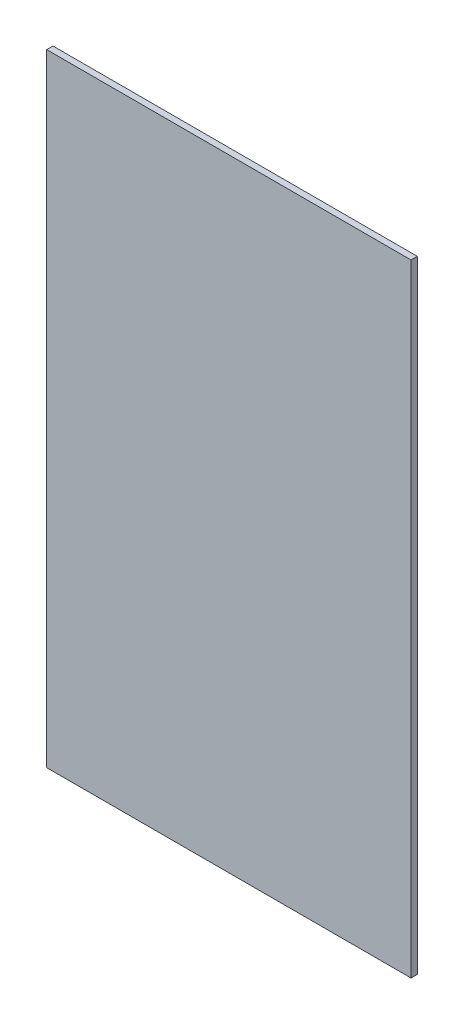
SolidWorks part; units mm, degrees
ref_plane "Front Plane" through (0, 0, 0) normal (0, 0, 1) x (1, 0, 0)
ref_plane "Top Plane" through (0, 0, 0) normal (0, 1, 0) x (1, 0, 0)
ref_plane "Right Plane" through (0, 0, 0) normal (1, 0, 0) x (0, 0, -1)
other "Configuration Table"
sketch "Sketch1" plane through (0, 0, 0) normal (0, 0, 1) x (1, 0, 0)
  line L1 (-29, 49.5) -> (29, 49.5)
  line L2 (-29, 49.5) -> (-29, -49.5)
  line L3 (-29, -49.5) -> (29, -49.5)
  line L4 (29, 49.5) -> (29, -49.5)
  line L5 (-29, 49.5) -> (29, -49.5) construction
  line L6 (-29, -49.5) -> (29, 49.5) construction
  point P0 (0, 0)
  dimension "D1" = 58
  dimension "D2" = 99
extrude "Boss-Extrude1" add sketch "Sketch1" along normal blind 1
